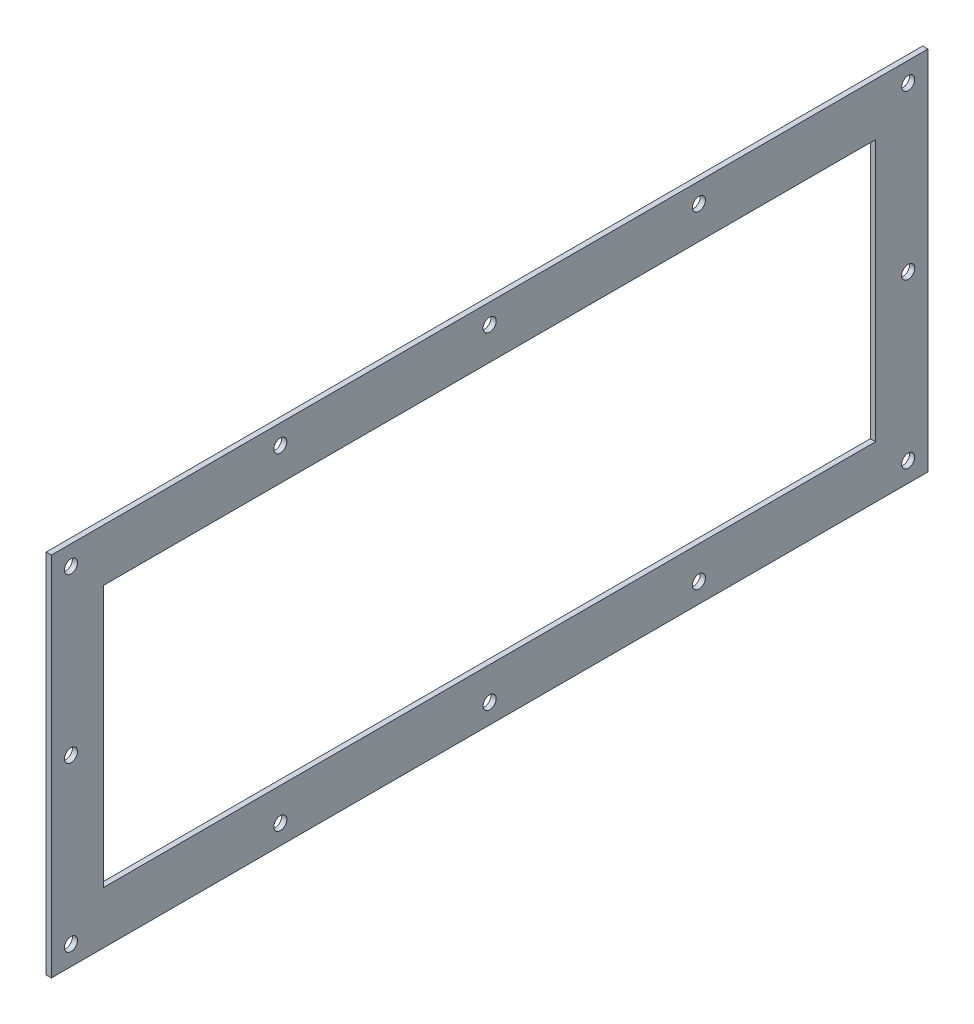
SolidWorks part; units mm, degrees
material "Q235"
ref_plane "前视基准面" through (0, 0, 0) normal (0, 0, 1) x (1, 0, 0)
ref_plane "上视基准面" through (0, 0, 0) normal (0, 1, 0) x (1, 0, 0)
ref_plane "右视基准面" through (0, 0, 0) normal (1, 0, 0) x (0, 0, -1)
sketch "草图1" plane through (0, 0, 0) normal (1, 0, 0) x (0, 0, -1)
  line L1 (-335, 140) -> (335, 140)
  line L2 (-335, 140) -> (-335, -140)
  line L3 (-335, -140) -> (335, -140)
  line L4 (335, 140) -> (335, -140)
  dimension "D1" = 670
  dimension "D2" = 335
  dimension "D3" = 280
  dimension "D4" = 140
extrude "拉伸-薄壁1" add sketch "草图1" along normal blind 4 thin
hole_wizard "Ø10.0 (10) 直径孔1" positions "草图3" profile "草图2" hole size "Ø10.0" standard "Gb" end condition through all
sketch "草图3" plane through (4, 0, 0) normal (1, 0, 0) x (0, 0, -1)
  line L0 (335, 140) -> (-335, 140) construction
  line L1 (-335, 140) -> (-335, -140) construction
  point P0 (-320, 125)
  dimension "D1" = 15
  dimension "D2" = 15
sketch "草图2" plane through (4, 125, 320) normal (0, 1, 0) x (0, 0, -1)
  line L0 (0, 0) -> (0, 4)
  line L1 (0, 4) -> (5, 4)
  line L2 (5, 4) -> (5, 0)
  line L5 (5, 0) -> (0, 0)
  line L11 (0, -6.35) -> (0, 107.95) construction
  dimension "通孔孔直径" = 10
  dimension "通孔孔深度" = 4
pattern_linear "阵列(线性)1" count 5 spacing 160 along (0, 0, -1) count 3 spacing 125 along (0, -1, 0) skipping (1, 1), (2, 1), (3, 1) of "Ø10.0 (10) 直径孔1"
